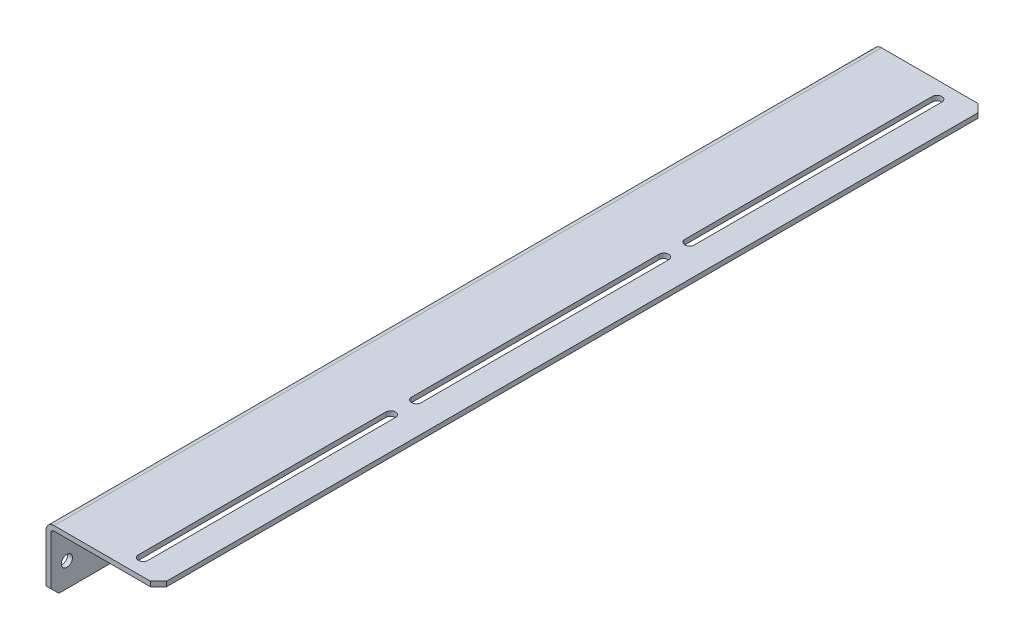
from build123d import *

# Parameters (mm, degrees)
EXTRUDE_1_DEPTH     = 515
SKETCH_3_R          = 3.5
CUT_EXTRUDE_1_DEPTH = 515
CHAMFER_1_SIZE      = 5
CUT_EXTRUDE_2_DEPTH = 515


with BuildPart() as part:
    # 草图1 → 凸台-拉伸1 (new body)
    with BuildSketch(Plane.XY):
        with BuildLine():
            Line((0, 0), (-65, 0))
            ThreePointArc((-65, 0), (-68.535533906, -1.464466094), (-70, -5))
            Line((-70, -5), (-70, -40))
            Line((-70, -40), (-67, -40))
            Line((-67, -40), (-67, -5))
            ThreePointArc((-67, -5), (-66.414213562, -3.585786438), (-65, -3))
            Line((-65, -3), (0, -3))
            Line((0, -3), (0, 0))
        make_face()
    extrude(amount=EXTRUDE_1_DEPTH)

    # 草图3 → 切除-拉伸1 (cut)
    with BuildSketch(Plane.ZY.offset(70)):
        with Locations((10, -25)):
            Circle(SKETCH_3_R)
        with Locations((70, -25)):
            Circle(SKETCH_3_R)
        with Locations((287.5, -25)):
            Circle(SKETCH_3_R)
        with Locations((180, -25)):
            Circle(SKETCH_3_R)
        with Locations((120, -25)):
            Circle(SKETCH_3_R)
        with Locations((227.5, -25)):
            Circle(SKETCH_3_R)
        with Locations(Location((445, -25, 0), (0, 0, 180))):
            Circle(SKETCH_3_R)
        with Locations(Location((505, -25, 0), (0, 0, 180))):
            Circle(SKETCH_3_R)
        with Locations(Location((395, -25, 0), (0, 0, 180))):
            Circle(SKETCH_3_R)
        with Locations(Location((335, -25, 0), (0, 0, 180))):
            Circle(SKETCH_3_R)
    extrude(amount=-CUT_EXTRUDE_1_DEPTH, mode=Mode.SUBTRACT)

    # 倒角1
    chamfer_1_edges = [part.edges().sort_by_distance(p)[0] for p in [
        (-68.5, -40, 0),
        (0, -1.5, 515),
        (-68.5, -40, 515),
        (0, -1.5, 0),
    ]]
    chamfer(chamfer_1_edges, length=CHAMFER_1_SIZE)

    # 草图4 → 切除-拉伸2 (cut)
    with BuildSketch(Plane(origin=(0, 0, 0), x_dir=(1, 0, 0), z_dir=(0, 1, 0))):
        with BuildLine():
            Line((-17, -10.5), (-17, -164.5))
            ThreePointArc((-17, -164.5), (-20, -167.5), (-23, -164.5))
            Line((-23, -164.5), (-23, -10.5))
            ThreePointArc((-23, -10.5), (-20, -7.5), (-17, -10.5))
        make_face()
        with BuildLine():
            Line((-17, -180.5), (-17, -334.5))
            ThreePointArc((-17, -334.5), (-20, -337.5), (-23, -334.5))
            Line((-23, -334.5), (-23, -180.5))
            ThreePointArc((-23, -180.5), (-20, -177.5), (-17, -180.5))
        make_face()
        with BuildLine():
            Line((-17, -504.5), (-17, -350.5))
            ThreePointArc((-17, -350.5), (-20, -347.5), (-23, -350.5))
            Line((-23, -350.5), (-23, -504.5))
            ThreePointArc((-23, -504.5), (-20, -507.5), (-17, -504.5))
        make_face()
    extrude(amount=-CUT_EXTRUDE_2_DEPTH, mode=Mode.SUBTRACT)


solid = part.part
